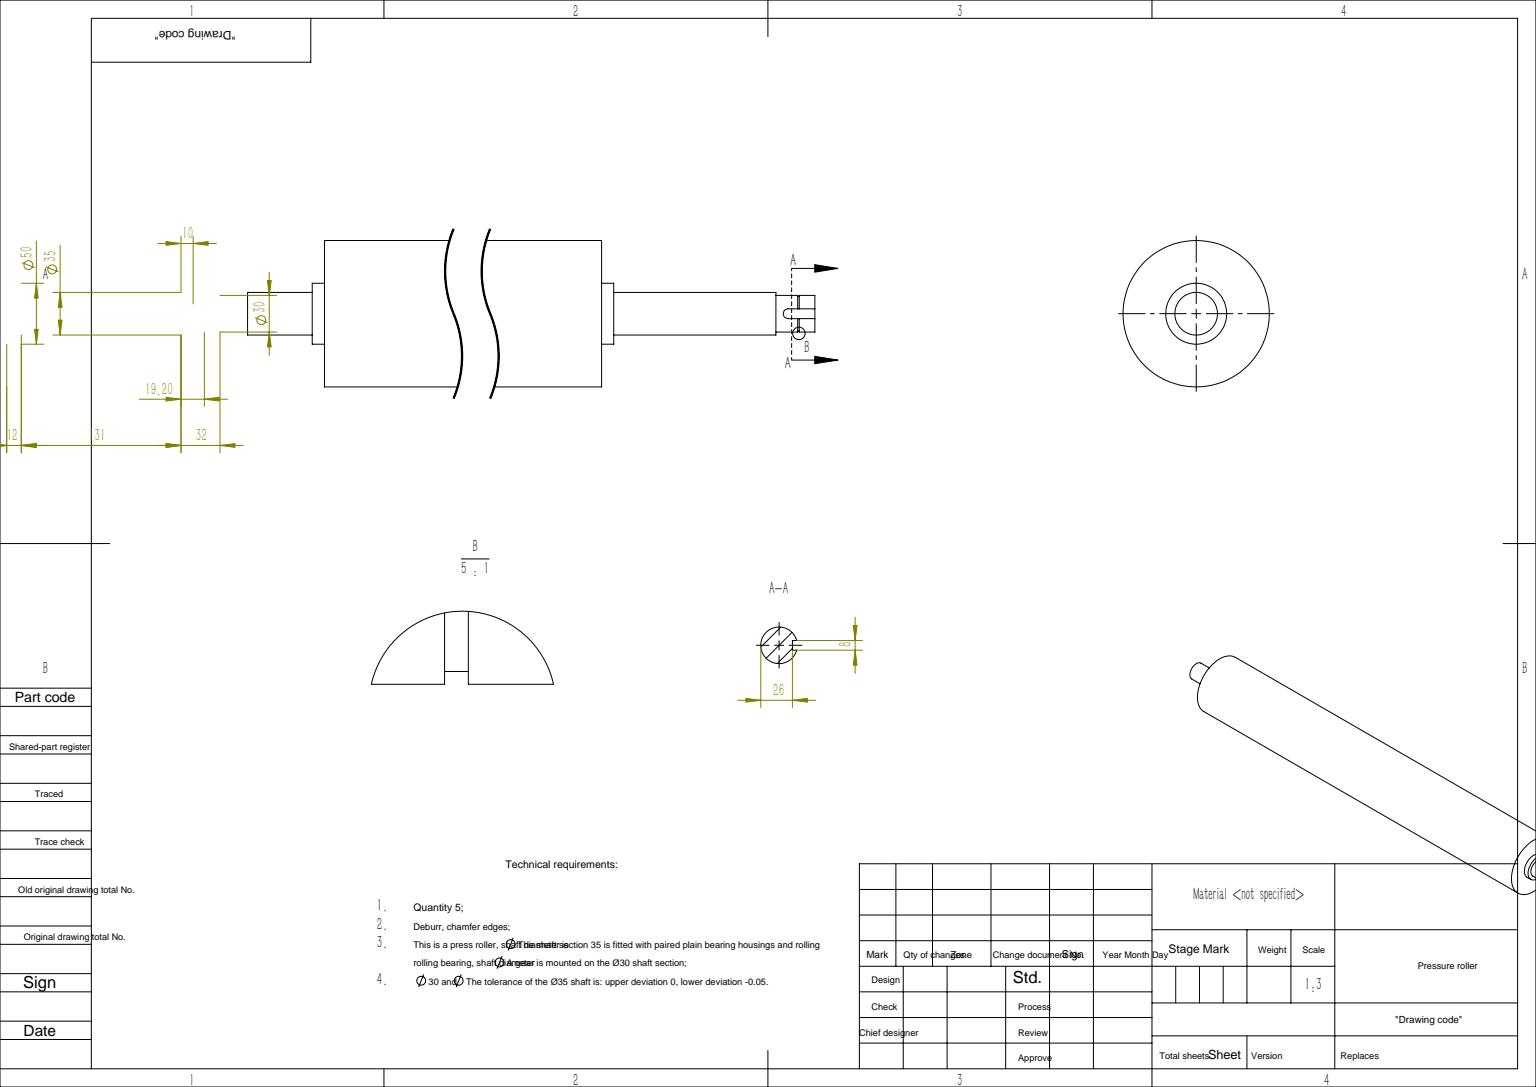
from build123d import *

# Parameters (mm, degrees)
CUT_EXTRUDE_1_DEPTH = 4
SKETCH_3_R          = 15
SKETCH_3_R_2        = 14.3
CUT_EXTRUDE_2_DEPTH = 1.3


with BuildPart() as part:
    # 草图1 → 旋转1 (revolve)
    with BuildSketch(Plane.XY, mode=Mode.PRIVATE) as revolve_1_sk:
        Polygon((0, 0), (0, 17.5), (53, 17.5), (53, 25), (63, 25), (63, 60), (913, 60), (913, 25), (923, 25), (923, 17.5), (1056, 17.5), (1056, 15), (1088, 15), (1088, 0), align=None)
    revolve(revolve_1_sk.sketch.rotate(Axis((1088, 0, 0), (-1, 0, 0)), 90), axis=Axis((1088, 0, 0), (-1, 0, 0)))

    # 草图2 → 切除-拉伸1 (cut)
    with BuildSketch(Plane(origin=(0, 15, 0), x_dir=(1, 0, 0), z_dir=(0, 1, 0))):
        with BuildLine():
            Line((1066, 4), (1098, 4))
            Line((1098, 4), (1098, -4))
            Line((1098, -4), (1066, -4))
            ThreePointArc((1066, -4), (1062, 0), (1066, 4))
        make_face()
    extrude(amount=-CUT_EXTRUDE_1_DEPTH, mode=Mode.SUBTRACT)

    # 草图3 → 切除-拉伸2 (cut)
    with BuildSketch(Plane(origin=(1075.2, 0, 0), x_dir=(0, 0, -1), z_dir=(1, 0, 0))):
        Circle(SKETCH_3_R)
        Circle(SKETCH_3_R_2, mode=Mode.SUBTRACT)
    extrude(amount=-CUT_EXTRUDE_2_DEPTH, mode=Mode.SUBTRACT)


solid = part.part
